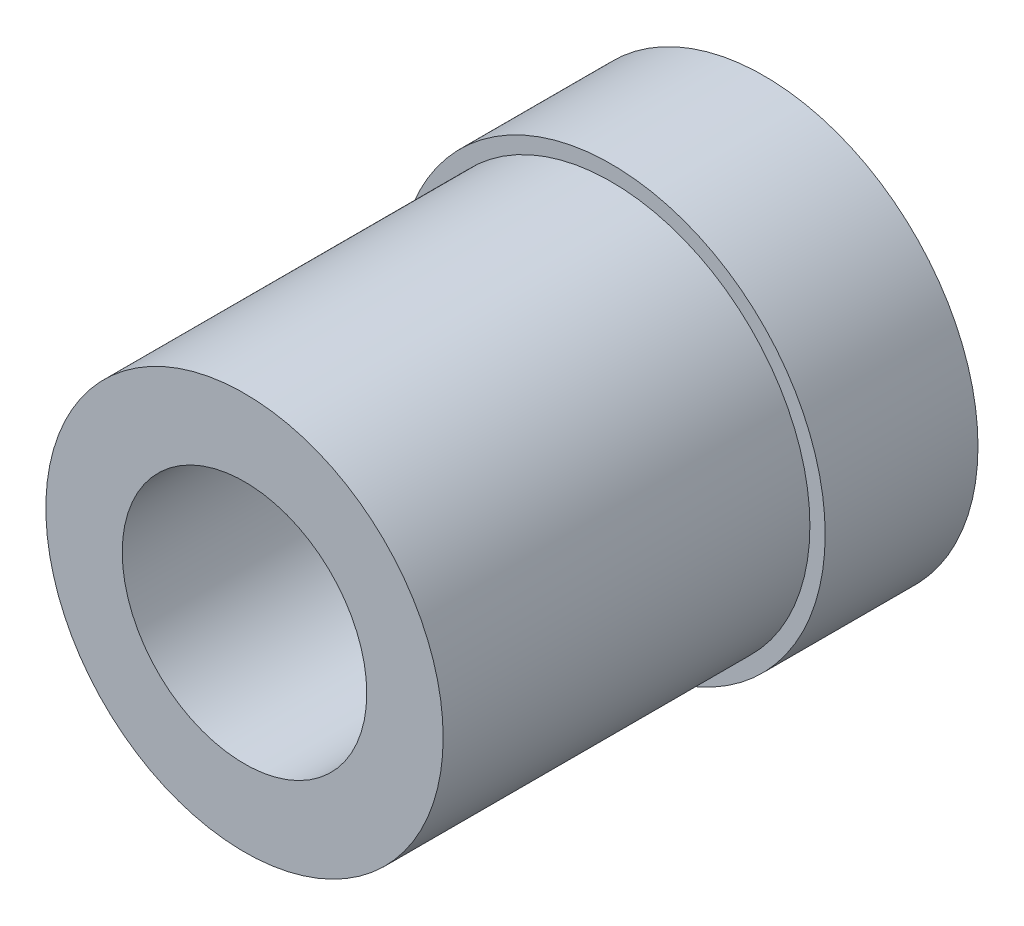
SolidWorks part; units mm, degrees
ref_plane "Front Plane" through (0, 0, 0) normal (0, 0, 1) x (1, 0, 0)
ref_plane "Top Plane" through (0, 0, 0) normal (0, 1, 0) x (1, 0, 0)
ref_plane "Right Plane" through (0, 0, 0) normal (1, 0, 0) x (0, 0, -1)
other "Configuration Table"
sketch "Sketch1" plane through (0, 0, 0) normal (0, 0, 1) x (1, 0, 0)
  circle A0 centre (0, 0) radius 7
  circle A1 centre (0, 0) radius 4
  dimension "D1" = 8
  dimension "D2" = 14
extrude "Boss-Extrude1" add sketch "Sketch1" along normal blind 5
sketch "Sketch2" plane through (0, 0, 5) normal (0, 0, 1) x (1, 0, 0)
  circle A0 centre (0, 0) radius 4
  circle A1 centre (0, 0) radius 6.5
  dimension "D1" = 13
extrude "Boss-Extrude2" add sketch "Sketch2" along normal blind 12
